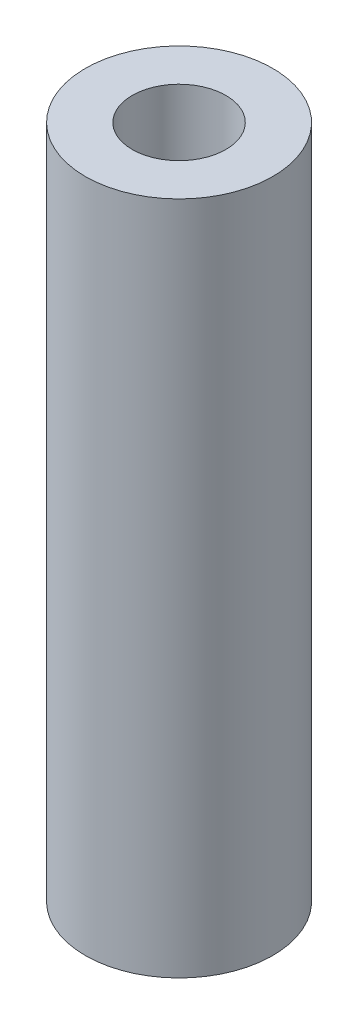
from build123d import *

# Parameters (mm, degrees)
SKETCH_1_R         = 2.5
EXTRUDE_1_DEPTH    = 18
HOLE_WIZARD_M3_1_D = 2.5


with BuildPart() as part:
    # 草图1 → 凸台-拉伸1 (new body)
    with BuildSketch(Plane(origin=(0, 0, 0), x_dir=(1, 0, 0), z_dir=(0, 1, 0))):
        with Locations(Location((0, 0, 0), (0, 0, 270))):
            Circle(SKETCH_1_R)
    extrude(amount=EXTRUDE_1_DEPTH)

    # M3 螺纹孔1 (through all)
    with Locations(Plane(origin=(0, 18, 0), x_dir=(1, 0, 0), z_dir=(0, 1, 0))):
        with Locations((0, 0)):
            Hole(HOLE_WIZARD_M3_1_D / 2)


solid = part.part
